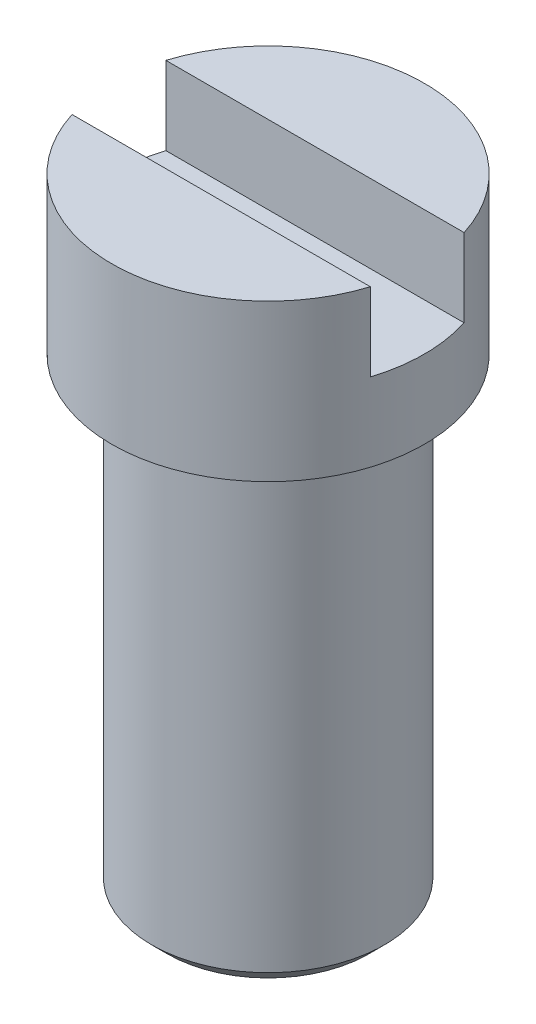
from build123d import *

# Parameters (mm, degrees)
SKETCH_1_R          = 7.45
EXTRUDE_1_DEPTH     = 30
SKETCH_2_R          = 10
EXTRUDE_2_DEPTH     = 10
SKETCH_4_W          = 50
SKETCH_4_H          = 6
CUT_EXTRUDE_2_DEPTH = 5
CHAMFER_1_SIZE      = 1


with BuildPart() as part:
    # 草图1 → 凸台-拉伸1 (new body)
    with BuildSketch(Plane(origin=(0, 0, 0), x_dir=(1, 0, 0), z_dir=(0, 1, 0))):
        with Locations(Location((0, 0, 0), (0, 0, 270))):
            Circle(SKETCH_1_R)
    extrude(amount=-EXTRUDE_1_DEPTH)

    # 草图2 → 凸台-拉伸2 (add)
    with BuildSketch(Plane(origin=(0, 0, 0), x_dir=(1, 0, 0), z_dir=(0, 1, 0))):
        with Locations(Location((0, 0, 0), (0, 0, 270))):
            Circle(SKETCH_2_R)
    extrude(amount=EXTRUDE_2_DEPTH)

    # 草图4 → 切除-拉伸2 (cut)
    with BuildSketch(Plane(origin=(0, 10, 0), x_dir=(1, 0, 0), z_dir=(0, 1, 0))):
        Rectangle(SKETCH_4_W, SKETCH_4_H)
    extrude(amount=-CUT_EXTRUDE_2_DEPTH, mode=Mode.SUBTRACT)

    # 倒角1
    chamfer_1_edges = [part.edges().sort_by_distance(p)[0] for p in [
        (0, -30, -7.45),
    ]]
    chamfer(chamfer_1_edges, length=CHAMFER_1_SIZE)


solid = part.part
